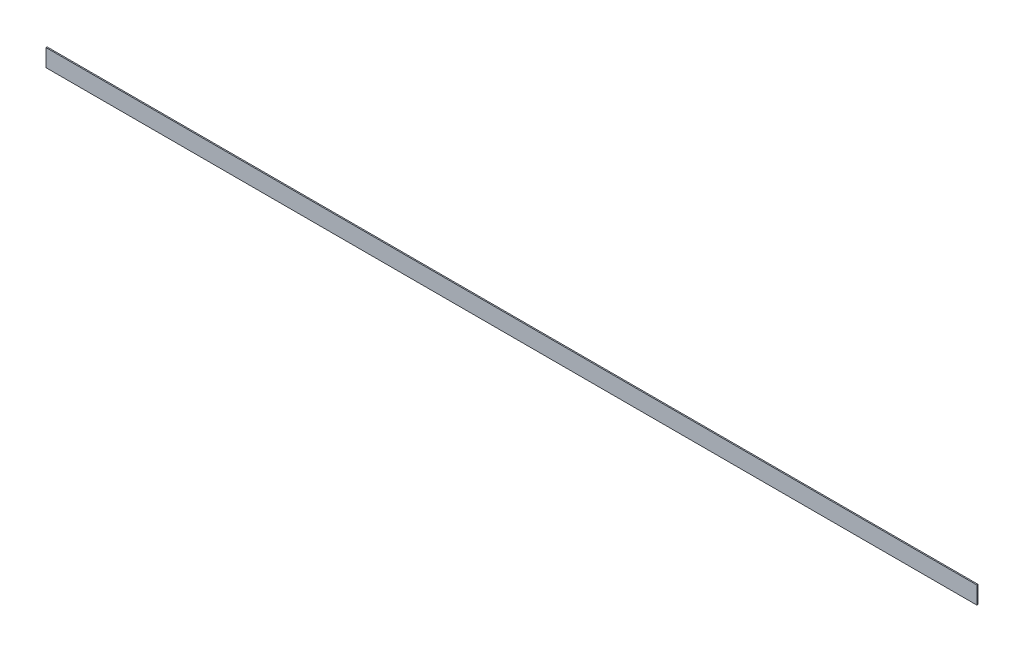
from build123d import *

# Parameters (mm, degrees)
SKETCH1_W           = 16000
SKETCH1_H           = 300
BOSS_EXTRUDE1_DEPTH = 20


with BuildPart() as part:
    # Sketch1 → Boss-Extrude1 (new body)
    with BuildSketch(Plane.XY):
        Rectangle(SKETCH1_W, SKETCH1_H)
    extrude(amount=BOSS_EXTRUDE1_DEPTH)


solid = part.part
